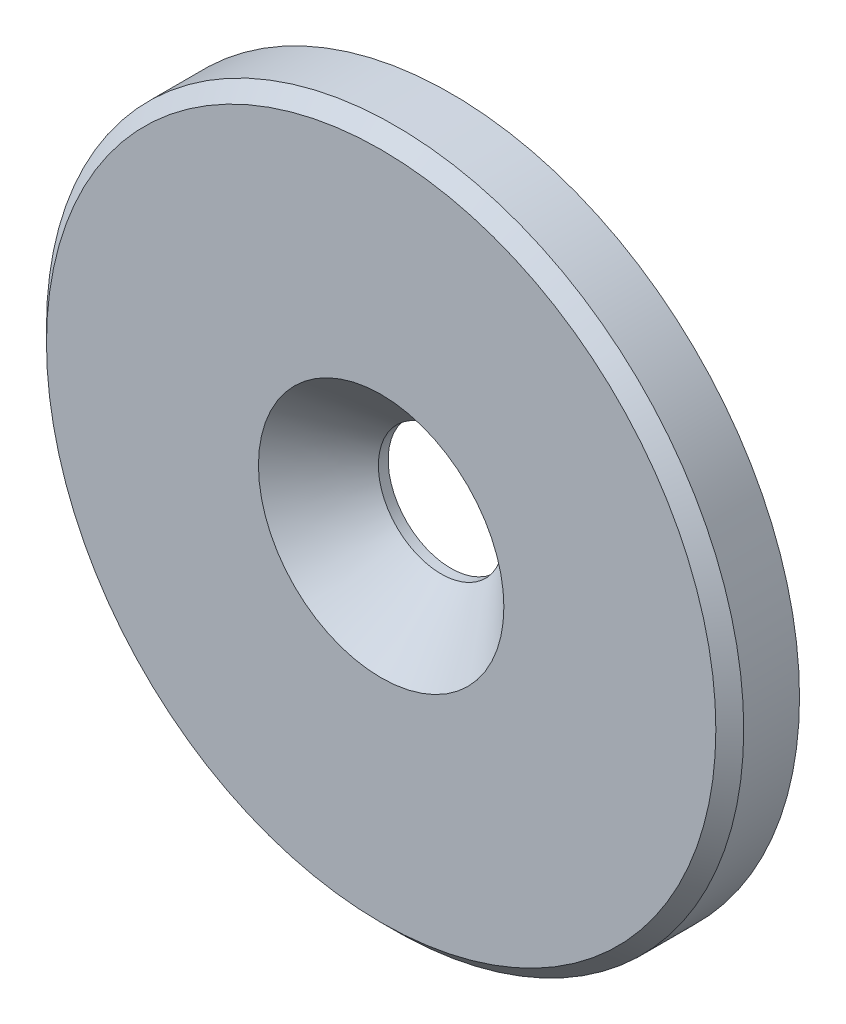
SolidWorks part; units mm, degrees
material "Q235-A"
ref_plane "前视基准面" through (0, 0, 0) normal (0, 0, 1) x (1, 0, 0)
ref_plane "上视基准面" through (0, 0, 0) normal (0, 1, 0) x (1, 0, 0)
ref_plane "右视基准面" through (0, 0, 0) normal (1, 0, 0) x (0, 0, -1)
sketch "草图1" plane through (0, 0, 0) normal (0, 0, 1) x (1, 0, 0)
  circle A0 centre (0, 0) radius 25
  dimension "D1" = 50
extrude "凸台-拉伸1" add sketch "草图1" along normal blind 5
hole_wizard "打孔尺寸(%根据)内六角花形半沉头螺钉的类型1" positions "草图2" profile "草图3" countersink size "M8" standard "GB" end condition through all
sketch "草图2" plane through (0, 0, 5) normal (0, 0, 1) x (1, 0, 0)
  point P0 (0, 0)
sketch "草图3" plane through (0, 0, 5) normal (1, 0, 0) x (0, -1, 0)
  line L0 (0, 0) -> (0, 5)
  line L1 (0, 5) -> (4.5, 5)
  line L2 (4.5, 5) -> (4.5, 4.3)
  line L3 (4.5, 4.3) -> (8.8, 0)
  line L5 (8.8, 0) -> (0, 0)
  line L6 (-4.5, 4.3) -> (-8.8, 0) construction
  line L11 (0, -6.35) -> (0, 107.95) construction
  dimension "通孔孔直径" = 9
  dimension "通孔孔深度" = 5
  dimension "近端锥形沉头孔直径" = 17.6
  dimension "近端锥形沉头孔角度" = 90
chamfer "倒角1" distance 1 angle 45 1 edges at (25, 0, 5)
